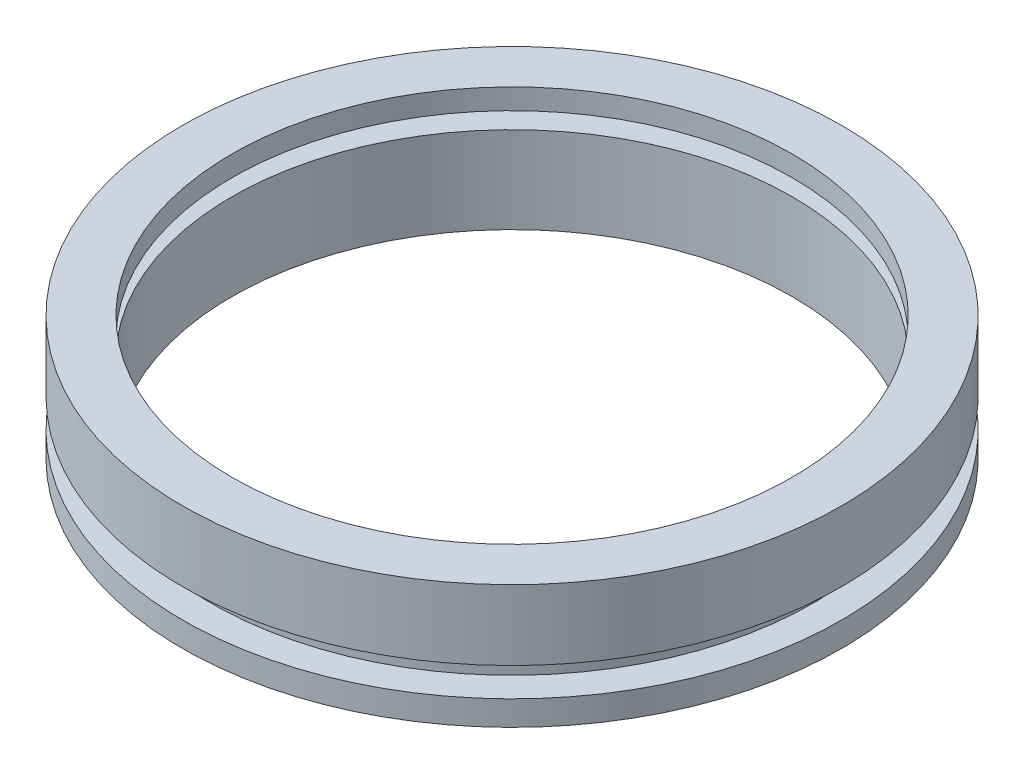
from build123d import *


with BuildPart() as part:
    # 草图1 → 旋转1 (revolve)
    with BuildSketch(Plane.XY, mode=Mode.PRIVATE) as revolve_1_sk:
        Polygon((0, 0), (-6, 0), (-6, 3), (-2.5, 3), (-2.5, 6.5), (-6, 6.5), (-6, 15), (0, 15), (0, 12.5), (-3.5, 12.5), (-3.5, 10.5), (0, 10.5), align=None)
    revolve(revolve_1_sk.sketch.rotate(Axis((34, 0, 0), (0, 1, 0)), 270), axis=Axis((34, 0, 0), (0, 1, 0)))


solid = part.part
